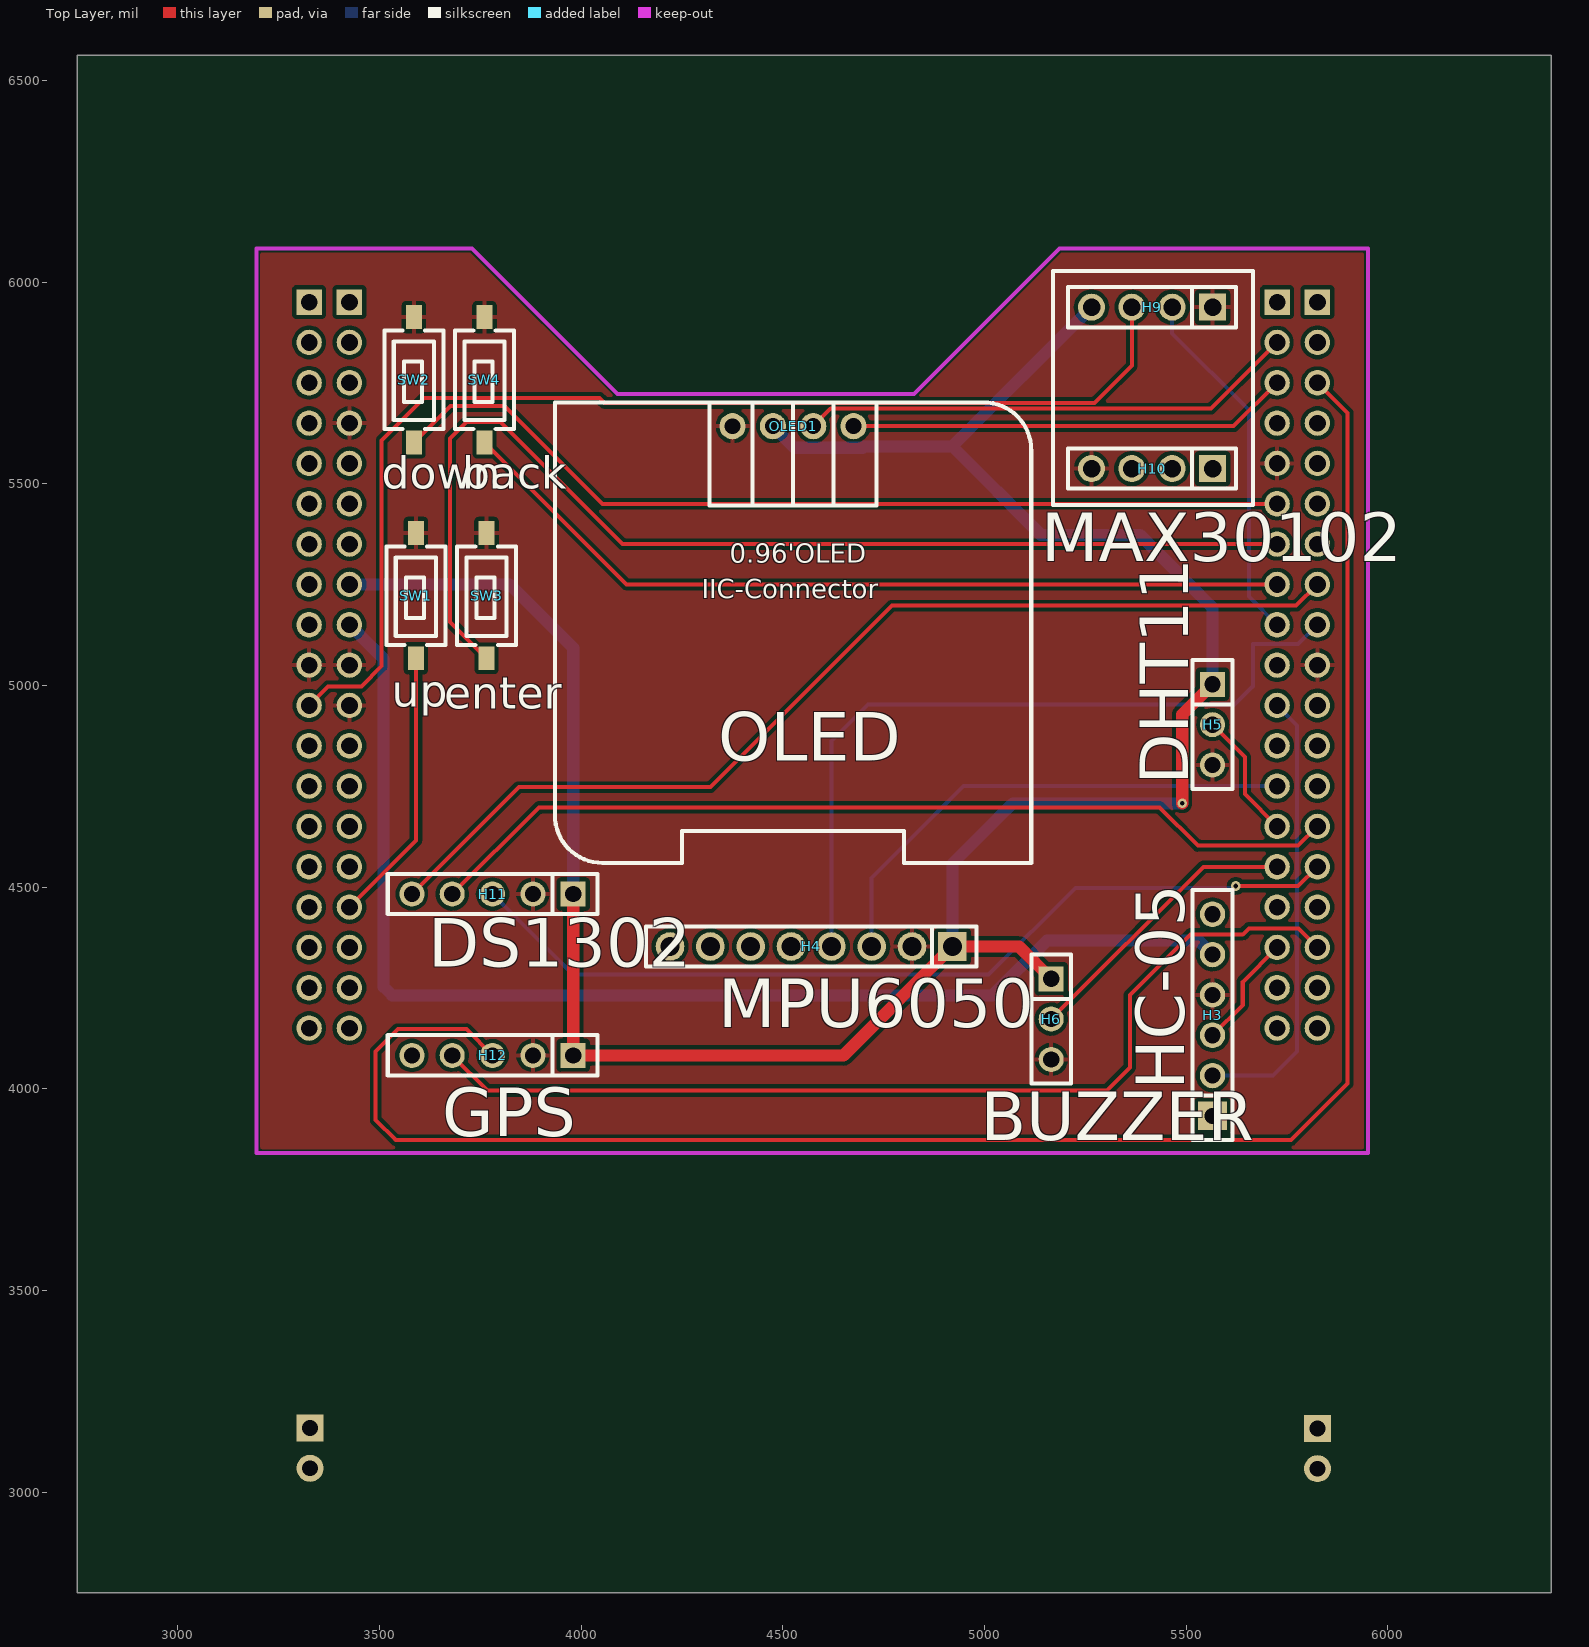
[diagram p0: Top Layer view]
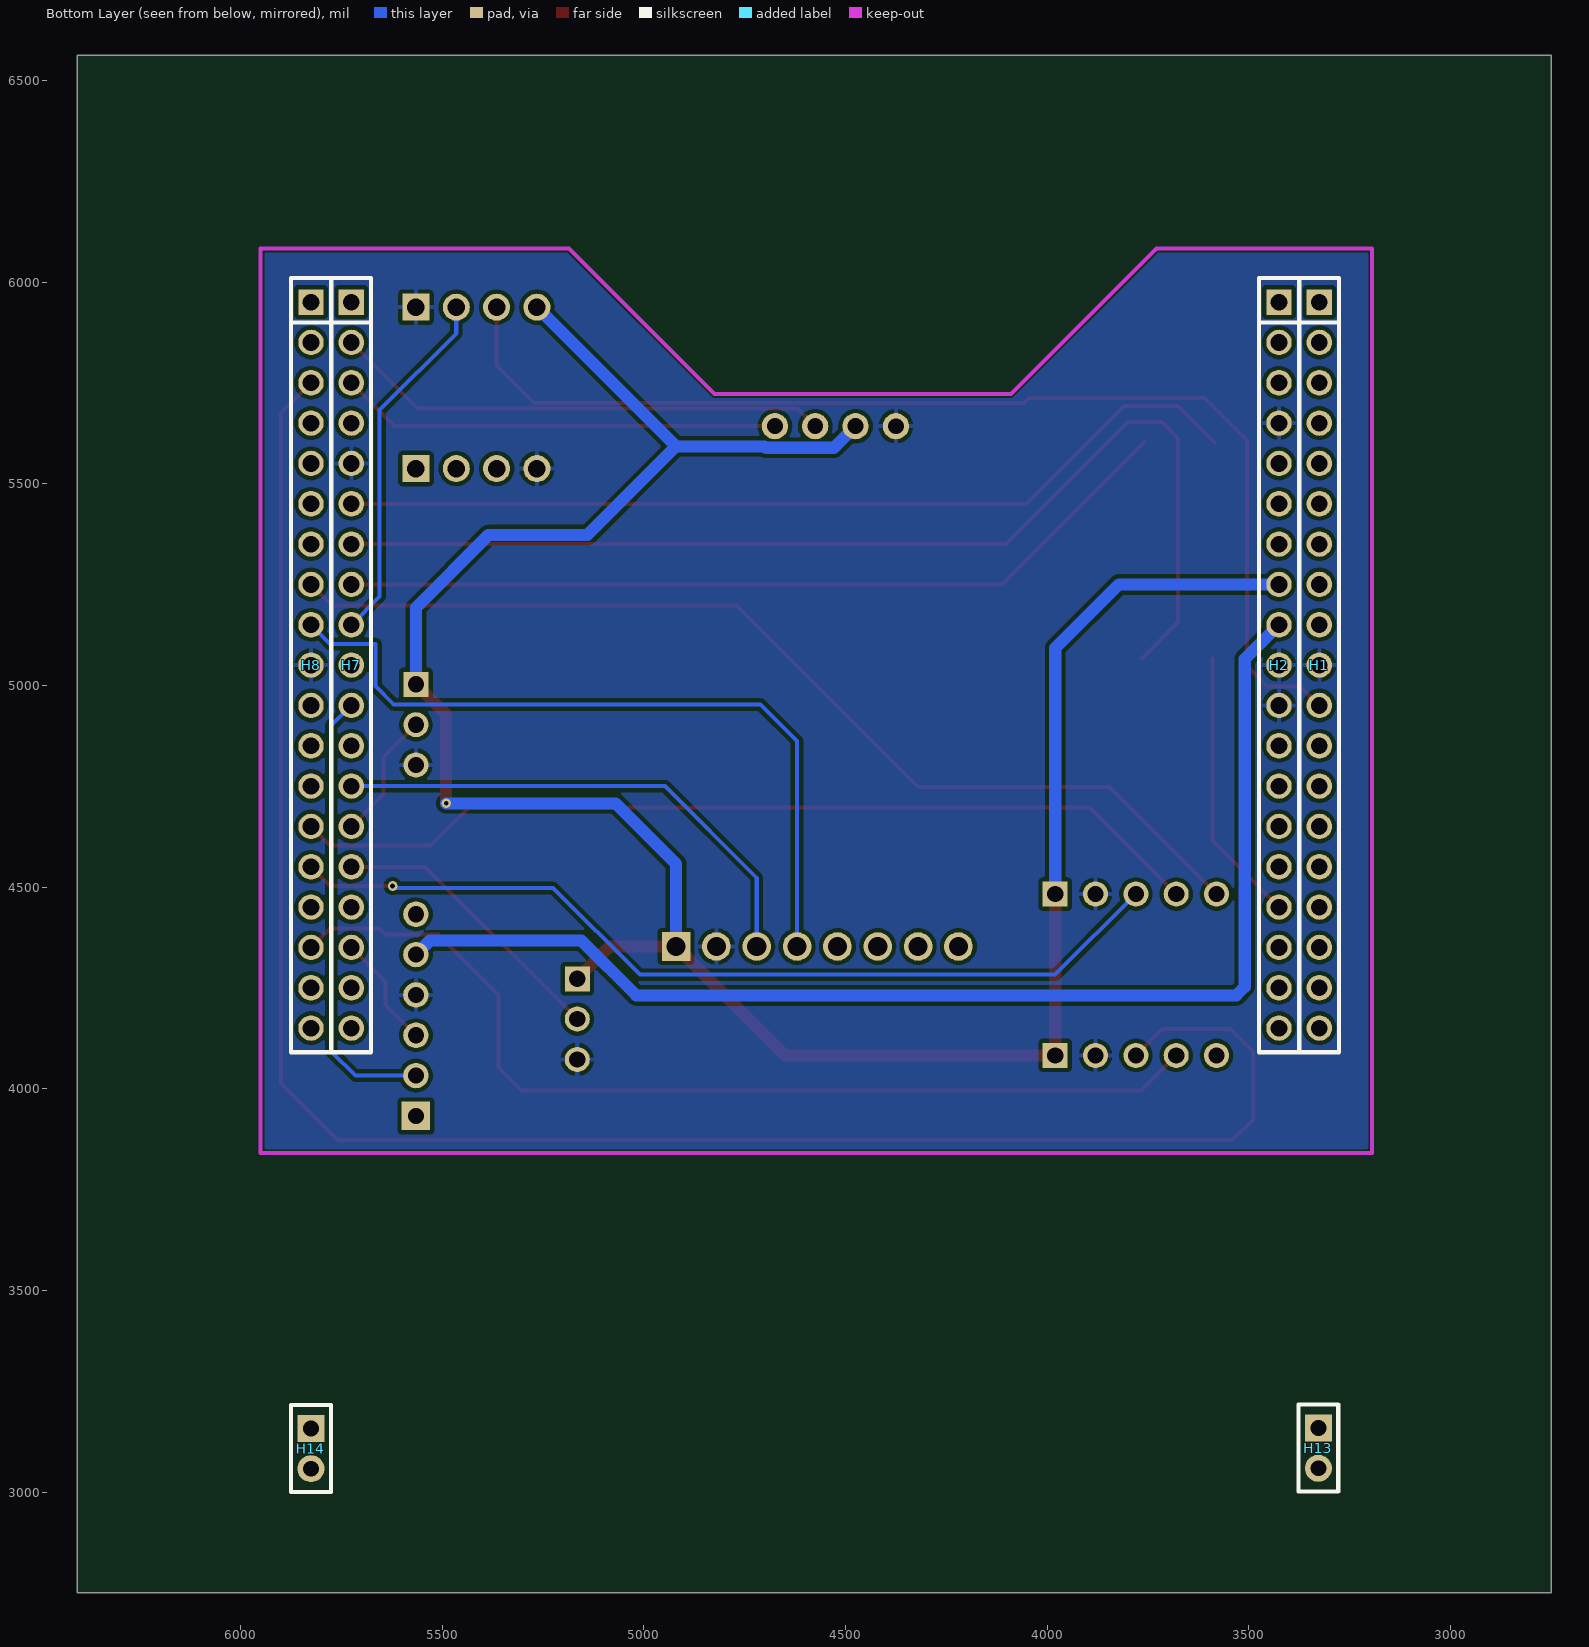
[diagram p1: Bottom Layer view, seen from below]
# Altium PCB MISC49932.pcbdoc
Units mil, origin at the board's own origin, x right, y up, seen from the top; angles counter-clockwise.
Board outline 3655 x 3812.56 mil, 2 copper layers (Top Layer, Bottom Layer), stack 62.206 mil thick; 19 components, 75 nets, 130 pads, 2 vias.

## Layer stack, top to bottom
Top Solder Mask Layer: solder mask 0.394, Dk 3.3
Top Layer: signal copper 1.379
Dielectric1: surface 59.449, FR4, Dk 4.5
Bottom Layer: signal copper 1.378
Bottom Solder Mask Layer: solder mask 0.394, Dk 3.3

## Board outline
6405,2750 2750,2750 2750,6562.56 6405,6562.56

## Design rules (kind name [scope] priority, off if disabled: settings)
BoardOutlineClearance copperThickness2oz_1 [All] p2 off: genericclearance=7.99 ignorepadtopadclearanceinfootprint=FALSE except(0: Arc-SplitContinuation Track-SplitContinuation SMDPad-SplitContinuation THPad-SplitContinuation Via-SplitContinuation Fill-SplitContinuation Region-SplitContinuation Poly-SplitContinuation Text-SplitContinuation Hole-SplitContinuation; 5.98: Arc-CutoutEdge SMDPad-CutoutEdge THPad-CutoutEdge Via-CutoutEdge Fill-CutoutEdge Region-CutoutEdge Text-CutoutEdge; 6.93: Hole-OutlineEdge Hole-CutoutEdge; 10: Poly-OutlineEdge Poly-CutoutEdge; 11.81: Arc-OutlineEdge Track-OutlineEdge SMDPad-OutlineEdge THPad-OutlineEdge Via-OutlineEdge Fill-OutlineEdge Region-OutlineEdge Text-OutlineEdge Track-CutoutEdge)
BoardOutlineClearance Plane_innerPlane_1 [All] p4 off: genericclearance=4.02 ignorepadtopadclearanceinfootprint=FALSE except(0: Arc-SplitContinuation Track-SplitContinuation SMDPad-SplitContinuation THPad-SplitContinuation Via-SplitContinuation Fill-SplitContinuation Region-SplitContinuation Poly-SplitContinuation Text-SplitContinuation Hole-SplitContinuation; 6: SMDPad-CutoutEdge THPad-CutoutEdge Via-CutoutEdge Fill-CutoutEdge Region-CutoutEdge Text-CutoutEdge; 6.93: Hole-OutlineEdge Hole-CutoutEdge; 10: Poly-OutlineEdge Poly-CutoutEdge; 11.8: Arc-OutlineEdge Track-OutlineEdge SMDPad-OutlineEdge THPad-OutlineEdge Via-OutlineEdge Fill-OutlineEdge Region-OutlineEdge Text-OutlineEdge; 11.81: Arc-CutoutEdge Track-CutoutEdge)
BoardOutlineClearance Copper_copperRegion_1 [All] p6 off: genericclearance=4.02 ignorepadtopadclearanceinfootprint=FALSE except(0: Arc-SplitContinuation Track-SplitContinuation SMDPad-SplitContinuation THPad-SplitContinuation Via-SplitContinuation Fill-SplitContinuation Region-SplitContinuation Poly-SplitContinuation Text-SplitContinuation Hole-SplitContinuation; 6: SMDPad-CutoutEdge THPad-CutoutEdge Via-CutoutEdge Fill-CutoutEdge Region-CutoutEdge Text-CutoutEdge; 6.93: Hole-OutlineEdge Hole-CutoutEdge; 10: Poly-OutlineEdge Poly-CutoutEdge; 11.8: Arc-OutlineEdge Track-OutlineEdge SMDPad-OutlineEdge THPad-OutlineEdge Via-OutlineEdge Fill-OutlineEdge Region-OutlineEdge Text-OutlineEdge; 11.81: Arc-CutoutEdge Track-CutoutEdge)
BoardOutlineClearance Copper_copperRegion_copperThickness1oz_1 [All] p8 off: genericclearance=4.02 ignorepadtopadclearanceinfootprint=FALSE except(0: Arc-SplitContinuation Track-SplitContinuation SMDPad-SplitContinuation THPad-SplitContinuation Via-SplitContinuation Fill-SplitContinuation Region-SplitContinuation Poly-SplitContinuation Text-SplitContinuation Hole-SplitContinuation; 6: SMDPad-CutoutEdge THPad-CutoutEdge Via-CutoutEdge Fill-CutoutEdge Region-CutoutEdge Text-CutoutEdge; 6.93: Hole-OutlineEdge Hole-CutoutEdge; 10: Poly-OutlineEdge Poly-CutoutEdge; 11.8: Arc-OutlineEdge Track-OutlineEdge SMDPad-OutlineEdge THPad-OutlineEdge Via-OutlineEdge Fill-OutlineEdge Region-OutlineEdge Text-OutlineEdge; 11.81: Arc-CutoutEdge Track-CutoutEdge)
BoardOutlineClearance Copper_copperRegion_Copper_copperRegion_1 [All] p10 off: genericclearance=4.02 ignorepadtopadclearanceinfootprint=FALSE except(0: Arc-SplitContinuation Track-SplitContinuation SMDPad-SplitContinuation THPad-SplitContinuation Via-SplitContinuation Fill-SplitContinuation Region-SplitContinuation Poly-SplitContinuation Text-SplitContinuation Hole-SplitContinuation; 6: SMDPad-CutoutEdge THPad-CutoutEdge Via-CutoutEdge Fill-CutoutEdge Region-CutoutEdge Text-CutoutEdge; 6.93: Hole-OutlineEdge Hole-CutoutEdge; 10: Poly-OutlineEdge Poly-CutoutEdge; 11.8: Arc-OutlineEdge Track-OutlineEdge SMDPad-OutlineEdge THPad-OutlineEdge Via-OutlineEdge Fill-OutlineEdge Region-OutlineEdge Text-OutlineEdge; 11.81: Arc-CutoutEdge Track-CutoutEdge)
BoardOutlineClearance copperThickness1oz_1 [All] p12: genericclearance=4.02 ignorepadtopadclearanceinfootprint=FALSE except(0: Arc-SplitContinuation Track-SplitContinuation SMDPad-SplitContinuation THPad-SplitContinuation Via-SplitContinuation Fill-SplitContinuation Region-SplitContinuation Poly-SplitContinuation Text-SplitContinuation Hole-SplitContinuation; 6: SMDPad-CutoutEdge THPad-CutoutEdge Via-CutoutEdge Fill-CutoutEdge Region-CutoutEdge Text-CutoutEdge; 6.93: Hole-OutlineEdge Hole-CutoutEdge; 10: Poly-OutlineEdge Poly-CutoutEdge; 11.8: Arc-OutlineEdge Track-OutlineEdge SMDPad-OutlineEdge THPad-OutlineEdge Via-OutlineEdge Fill-OutlineEdge Region-OutlineEdge Text-OutlineEdge; 11.81: Arc-CutoutEdge Track-CutoutEdge)
Clearance copperThickness2oz [All] p1 off: gap=7.99 ignorepadtopadclearanceinfootprint=FALSE except(5.98: SMDPad-Track SMDPad-SMDPad THPad-Track SMDPad-THPad THPad-THPad Track-Via SMDPad-Via THPad-Via Via-Via Fill-Track Region-Track Fill-SMDPad Region-SMDPad Fill-THPad Region-THPad Fill-Via Region-Via Fill-Fill Fill-Region Region-Region Arc-Track Arc-SMDPad Arc-THPad Arc-Via Fill-Arc Region-Arc Arc-Arc Text-Track SMDPad-Text Text-THPad Text-Via Fill-Text Region-Text Arc-Text Text-Text; 6.93: Hole-Track Hole-SMDPad Hole-THPad Hole-Via Fill-Hole Region-Hole Hole-Arc Hole-Text; 10: Poly-Track Poly-SMDPad Poly-THPad Poly-Via Poly-Fill Poly-Region Poly-Poly Poly-Arc Poly-Text Poly-Hole)
Clearance Plane_innerPlane [All] p3 off: gap=4.02 ignorepadtopadclearanceinfootprint=FALSE except(5.98: SMDPad-Track SMDPad-SMDPad THPad-Track SMDPad-THPad THPad-THPad Track-Via SMDPad-Via THPad-Via Via-Via Fill-Track Region-Track Fill-SMDPad Region-SMDPad Fill-THPad Region-THPad Fill-Via Region-Via Fill-Fill Fill-Region Region-Region; 6: Arc-Track Arc-SMDPad Arc-THPad Arc-Via Fill-Arc Region-Arc Arc-Arc Text-Track SMDPad-Text Text-THPad Text-Via Fill-Text Region-Text Arc-Text Text-Text; 6.93: Hole-Track Hole-SMDPad Hole-THPad Hole-Via Fill-Hole Region-Hole Hole-Arc Hole-Text; 10: Poly-Track Poly-SMDPad Poly-THPad Poly-Via Poly-Fill Poly-Region Poly-Poly Poly-Arc Poly-Text Poly-Hole)
Clearance Copper_copperRegion [All] p5 off: gap=4.02 ignorepadtopadclearanceinfootprint=FALSE except(5.98: SMDPad-Track SMDPad-SMDPad THPad-Track SMDPad-THPad THPad-THPad Track-Via SMDPad-Via THPad-Via Via-Via Fill-Track Region-Track Fill-SMDPad Region-SMDPad Fill-THPad Region-THPad Fill-Via Region-Via Fill-Fill Fill-Region Region-Region; 6: Arc-Track Arc-SMDPad Arc-THPad Arc-Via Fill-Arc Region-Arc Arc-Arc Text-Track SMDPad-Text Text-THPad Text-Via Fill-Text Region-Text Arc-Text Text-Text; 6.93: Hole-Track Hole-SMDPad Hole-THPad Hole-Via Fill-Hole Region-Hole Hole-Arc Hole-Text; 10: Poly-Track Poly-SMDPad Poly-THPad Poly-Via Poly-Fill Poly-Region Poly-Poly Poly-Arc Poly-Text Poly-Hole)
Clearance Copper_copperRegion_copperThickness1oz [All] p7 off: gap=4.02 ignorepadtopadclearanceinfootprint=FALSE except(5.98: SMDPad-Track SMDPad-SMDPad THPad-Track SMDPad-THPad THPad-THPad Track-Via SMDPad-Via THPad-Via Via-Via Fill-Track Region-Track Fill-SMDPad Region-SMDPad Fill-THPad Region-THPad Fill-Via Region-Via Fill-Fill Fill-Region Region-Region; 6: Arc-Track Arc-SMDPad Arc-THPad Arc-Via Fill-Arc Region-Arc Arc-Arc Text-Track SMDPad-Text Text-THPad Text-Via Fill-Text Region-Text Arc-Text Text-Text; 6.93: Hole-Track Hole-SMDPad Hole-THPad Hole-Via Fill-Hole Region-Hole Hole-Arc Hole-Text; 10: Poly-Track Poly-SMDPad Poly-THPad Poly-Via Poly-Fill Poly-Region Poly-Poly Poly-Arc Poly-Text Poly-Hole)
Clearance Copper_copperRegion_Copper_copperRegion [All] p9 off: gap=4.02 ignorepadtopadclearanceinfootprint=FALSE except(5.98: SMDPad-Track SMDPad-SMDPad THPad-Track SMDPad-THPad THPad-THPad Track-Via SMDPad-Via THPad-Via Via-Via Fill-Track Region-Track Fill-SMDPad Region-SMDPad Fill-THPad Region-THPad Fill-Via Region-Via Fill-Fill Fill-Region Region-Region; 6: Arc-Track Arc-SMDPad Arc-THPad Arc-Via Fill-Arc Region-Arc Arc-Arc Text-Track SMDPad-Text Text-THPad Text-Via Fill-Text Region-Text Arc-Text Text-Text; 6.93: Hole-Track Hole-SMDPad Hole-THPad Hole-Via Fill-Hole Region-Hole Hole-Arc Hole-Text; 10: Poly-Track Poly-SMDPad Poly-THPad Poly-Via Poly-Fill Poly-Region Poly-Poly Poly-Arc Poly-Text Poly-Hole)
Clearance copperThickness1oz [All] p11: gap=4.02 ignorepadtopadclearanceinfootprint=FALSE except(5.98: SMDPad-Track SMDPad-SMDPad THPad-Track SMDPad-THPad THPad-THPad Track-Via SMDPad-Via THPad-Via Via-Via Fill-Track Region-Track Fill-SMDPad Region-SMDPad Fill-THPad Region-THPad Fill-Via Region-Via Fill-Fill Fill-Region Region-Region; 6: Arc-Track Arc-SMDPad Arc-THPad Arc-Via Fill-Arc Region-Arc Arc-Arc Text-Track SMDPad-Text Text-THPad Text-Via Fill-Text Region-Text Arc-Text Text-Text; 6.93: Hole-Track Hole-SMDPad Hole-THPad Hole-Via Fill-Hole Region-Hole Hole-Arc Hole-Text; 10: Poly-Track Poly-SMDPad Poly-THPad Poly-Via Poly-Fill Poly-Region Poly-Poly Poly-Arc Poly-Text Poly-Hole)
DiffPairsRouting differentialPair [All] p1: maxlimit=6 minlimit=6 mostfreqgap=6 toplayer_minwidth=5 toplayer_prefwidth=10 toplayer_maxwidth=100 toplayer_mingap=6 toplayer_prefgap=6 toplayer_maxgap=6 bottomlayer_minwidth=5 bottomlayer_prefwidth=10 bottomlayer_maxwidth=100 bottomlayer_mingap=6 bottomlayer_prefgap=6 bottomlayer_maxgap=6 maxuncoupledlength=10
HoleToHoleClearance otherClearance [All] p1: gap=11.81 allowstackedmicrovias=TRUE
Length netLength [All] p1: minlimit=0 maxlimit=0
PasteMaskExpansion pasteMaskExpansion [All] p1: expansion=0
PlaneConnect innerPlane [All] p1: planeconnectstyle=Relief reliefexpansion=20 reliefentries=4 reliefconductorwidth=10 reliefairgap=10
PolygonConnect copperRegion_copperThickness1oz [All] p1 off: connectstyle=Relief reliefconductorwidth=10 reliefentries=4 polygonreliefangle="90 Angle" airgapwidth=10 via.connectstyle=Relief via.reliefconductorwidth=10 via.reliefentries=4 via.polygonreliefangle="90 Angle" via.airgapwidth=10
PolygonConnect copperRegion_Copper_copperRegion [All] p2 off: connectstyle=Relief reliefconductorwidth=10 reliefentries=4 polygonreliefangle="90 Angle" airgapwidth=10 via.connectstyle=Relief via.reliefconductorwidth=10 via.reliefentries=4 via.polygonreliefangle="90 Angle" via.airgapwidth=10
PolygonConnect copperRegion [All] p3: connectstyle=Relief reliefconductorwidth=10 reliefentries=4 polygonreliefangle="90 Angle" airgapwidth=10 via.connectstyle=Relief via.reliefconductorwidth=10 via.reliefentries=4 via.polygonreliefangle="90 Angle" via.airgapwidth=10
RoutingVias viaSize [All] p1: holewidth=12.01 width=24.02 viastyle="Through Hole" minholewidth=11.81 minwidth=19.68 maxholewidth=248.03 maxwidth=393.7
SolderMaskExpansion solderMaskExpansion [IsVia] p1: expansion=-1000 istentingtop=TRUE
SolderMaskExpansion solderMaskExpansion [All] p2: expansion=2 istentingtop=FALSE
Width copperThickness2oz_2 [All] p1 off: maxlimit=100 minlimit=8 preferedwidth=10
Width copperThickness1oz_2 [All] p2: maxlimit=100 minlimit=5 preferedwidth=10

## Components (designator, comment, footprint, x,y, rotation, side; value= is the part's Value field where it differs from the comment)
H1 "C2897382" HDR-TH_19P-P2.54-V-F 3325.16,5050.22 r270 bottom locked
H2 "C2897382" HDR-TH_19P-P2.54-V-F 3425.16,5050.22 r270 bottom locked
H3 "" HDR-TH_6P-P2.54-V-F 5565,4182.56 r90 top
H4 "" HDR-TH_8P-P2.54-V-F-1 4570,4352.56 r180 top
H5 "" HDR-TH_3P-P2.54-V-F 5565,4902.56 r270 top
H6 "" HDR-TH_3P-P2.54-V-F 5165,4172.56 r270 top
H7 "C2897382" HDR-TH_19P-P2.54-V-F 5725.16,5050.22 r270 bottom locked
H8 "C2897382" HDR-TH_19P-P2.54-V-F 5825.16,5050.22 r270 bottom locked
H9 "" HDR-TH_4P-P2.54-V-F 5415,5937.56 r180 top
H10 "" HDR-TH_4P-P2.54-V-F 5415,5537.56 r180 top
H11 "" HDR-TH_5P-P2.54-V-F 3780,4482.56 r180 top
H12 "" HDR-TH_5P-P2.54-V-F 3780,4082.56 r180 top
H13 "" HDR-TH_2P-P2.54-V-F 3327.44,3108.94 r270 bottom locked
H14 "" HDR-TH_2P-P2.54-V-F 5825.32,3107.87 r270 bottom locked
OLED1 "" 0.96OLED_4P 4525,5642.56 r0 top
SW1 "" Key_SMD_3.6x6.1x2.5 3590,5222.56 r90 top
SW2 "" Key_SMD_3.6x6.1x2.5 3585,5757.56 r90 top
SW3 "" Key_SMD_3.6x6.1x2.5 3765,5222.56 r90 top
SW4 "" Key_SMD_3.6x6.1x2.5 3760,5757.56 r90 top

## Footprints (in the part's own frame and the unit in brackets; to place one, negate y for a bottom-side part, rotate by r counter-clockwise, add the part's x,y. Pads: shape width x height; smd on the part's side, far side on the other; paste and mask are expansions set on the pad)
0.96OLED_4P [mm]
  round 1.65 hole 1 copper offset 0,0: 1(-3.81,-0.001) 2(-1.27,0.002) 3(1.27,0.002) 4(3.81,0.002)
  silkscreen extent -15,-27.5 15,1.5
HDR-TH_2P-P2.54-V-F [mm]
  rect 1.7x1.7 hole 1: 1(-1.27,0)
  round 1.7 hole 1: 2(1.27,0)
  silkscreen extent -2.74,-1.25 2.74,1.25
HDR-TH_3P-P2.54-V-F [mil]
  rect 62x62 hole 40.16: 1(-100,0)
  round 62 hole 40.16: 2(0,0) 3(100,0)
  silkscreen extent -160,-49 160,49
HDR-TH_4P-P2.54-V-F [mm]
  rect 1.7x1.7 hole 1.1: 1(-3.81,0)
  round 1.7 hole 1.1: 2(-1.27,0) 3(1.27,0) 4(3.81,0)
  silkscreen extent -5.29,-1.27 5.29,1.27
HDR-TH_5P-P2.54-V-F [mil]
  rect 62x62 hole 40.16: 1(-200,0)
  round 62 hole 40.16: 2(-100,0) 3(0,0) 4(100,0) 5(200,0)
  silkscreen extent -260,-50 260,50
HDR-TH_6P-P2.54-V-F [mm]
  rect 1.8x1.8 hole 1.02: 1(-6.35,0)
  round 1.6 hole 1.02: 2(-3.81,0) 3(-1.27,0) 4(1.27,0) 5(3.81,0) 6(6.35,0)
  silkscreen extent -7.87,-1.25 7.87,1.25
HDR-TH_8P-P2.54-V-F-1 [mm]
  rect 1.8x1.8 hole 1.2: 1(-8.89,0)
  round 1.8 hole 1.2: 2(-6.35,0) 3(-3.81,0) 4(-1.27,0) 5(1.27,0) 6(3.81,0) 7(6.35,0) 8(8.89,0)
  silkscreen extent -10.41,-1.25 10.41,1.25
HDR-TH_19P-P2.54-V-F [mm]
  rect 1.6x1.6 hole 1.05: 1(-22.86,0)
  round 1.6 hole 1.05: 2(-20.32,0) 3(-17.78,0) 4(-15.24,0) 5(-12.7,0) 6(-10.16,0) 7(-7.62,0) 8(-5.08,0) 9(-2.54,0) 10(0,0) 11(2.54,0) 12(5.08,0) 13(7.62,0) 14(10.16,0) 15(12.7,0) 16(15.24,0) 17(17.78,0) 18(20.32,0) 19(22.86,0)
  silkscreen extent -24.38,-1.25 24.38,1.25
Key_SMD_3.6x6.1x2.5 [mil]
  rect 59.1x39.4 smd paste+0 mask+2: 1(-155.5,0) 2(155.5,0)
  silkscreen extent -122,-73 122,73

## Via types
v1: diameter 24.02, hole 12, Top Layer to Bottom Layer, 2 vias

## Nets (pads, with @x,y where several pads share a name; then routed paths per layer and width w, separated by ;. In a path a pad name is that pad's centre, name@x,y a point inside that pad or via, vN(x,y) a via of type N, cw(c..) or ccw(c..) an arc to the next point about the centre after c; other vN are vias at no path point)
+3V3: H2.8 H4.1 H5.1 H6.1 H9.4 H11.1 H12.1 OLED1.2 | length 6080.5
  Top Layer w30: H11.1 H12.1 4650,4082.56 H4.1 5085,4352.56 H6.1 ; v1(5490,4707.56) 5490,4927.56 H5.1
  Bottom Layer w30: H2.8 3822.35,5250.22 3980,5092.56 H11.1 ; OLED1.2 4528.46,5589.15 4697.15,5589.15 4700.56,5592.56 4920,5592.56 ; H4.1 4920,4557.56 5070,4707.56 v1(5490,4707.56) ; H9.4 4920,5592.56 ; H5.1 5565,5192.56 5385,5372.56 5140,5372.56 4920,5592.56
+5V: H2.9 H3.5 | length 3067.5
  Bottom Layer w30: H2.9 3510,5065.38 3510,4252.56 3531.21,4231.35 5018.79,4231.35 5155,4367.56 5530,4367.56 H3.5
ADO: H4.7
AGND: H8.16
AVDD: H7.4
BOOT0: H1.4
CLK: H8.15 H11.3 | length 2238.8
  Top Layer w10: v1@5622.78,4502.56 5777.5,4502.56 H8.15
  Bottom Layer w10: H11.3 3980,4282.56 5010,4282.56 5225,4497.56 5617.78,4497.56 v1(5622.74,4502.52)
DAT: H8.14 H11.4 | length 2293.3
  Top Layer w10: H11.4 3895,4697.56 5433.54,4697.56 5528.54,4602.56 5777.5,4602.56 H8.14
E5V: H2.3
EN: H3.6
GND: H1.10 H2.4 H2.10 H2.11 H3.4 H4.2 H5.3 H6.3 H7.5 H8.10 H9.1 H10.4 H11.2 H12.2 OLED1.1 SW1.2 SW2.2 SW3.2 SW4.2
INT: H4.8
IOREF: H2.6
NC: H8.5
PA0: H2.14
PA1: H2.15
PA2: H7.18
PA3: H7.19
PA4: H2.16 SW1.1 | length 685.1
  Top Layer w10: H2.16 3590,4615.06 SW1.1
PA5: H7.6 SW2.1 | length 2278
  Top Layer w10: SW2.1 3675.5,5692.56 3810,5692.56 4052.35,5450.22 H7.6
PA6: H7.7 SW3.1 | length 2774.7
  Top Layer w10: SW3.1 3675,5157.06 3675,5612.56 3715,5652.56 3800,5652.56 4102.35,5350.22 H7.7
PA7: H7.8 SW4.1 | length 2110.9
  Top Layer w10: SW4.1 4111.85,5250.22 H7.8
PA8: H7.12
PA9: H3.2 H7.11 | length 1113.2
  Bottom Layer w10: H3.2 5715,4032.56 5775,4092.56 5775,4900.38 H7.11
PA10: H3.3 H7.17 | length 284
  Top Layer w10: H3.3 5640,4207.56 5640,4265.06 H7.17
PA11: H8.7
PA12: H8.6
PA13: H1.7
PA14: H1.8
PA15: H1.9
PB0: H2.17
PB1: H8.12
PB2: H8.11
PB3: H7.16
PB4: H5.2 H7.14 | length 318.7
  Top Layer w10: H5.2 5645,4822.56 5645,4730.38 H7.14
PB5: H6.2 H7.15 | length 716.6
  Top Layer w10: H6.2 5542.65,4550.22 H7.15
PB6: H7.9 H9.2 | length 895.1
  Bottom Layer w10: H9.2 5465,5872.56 5655,5682.56 5655,5220.38 H7.9
PB7: H1.11 H9.3 | length 2872.1
  Top Layer w10: H1.11 3372.5,4997.56 3455,4997.56 3505,5047.56 3505,5607.56 3610,5712.56 4045,5712.56 4057.47,5700.09 5272.53,5700.09 5365,5792.56 H9.3
PB8: H7.2 OLED1.3 | length 1236.2
  Top Layer w10: OLED1.3 4618.46,5686.08 5561.02,5686.08 H7.2
PB9: H7.3 OLED1.4 | length 1094.7
  Top Layer w10: OLED1.4 5617.55,5642.61 H7.3
PB10: H4.3 H7.13 | length 1269.5
  Bottom Layer w10: H4.3 4720,4522.56 4947.65,4750.22 H7.13
PB11: H4.4 H8.9 | length 1895.2
  Bottom Layer w10: H4.4 4620,4861.76 4710.8,4952.56 5620,4952.56 5665.28,4997.84 5665.28,5102.56 5777.5,5102.56 H8.9
PB12: H8.8 H11.5 | length 2563.1
  Top Layer w10: H11.5 3845,4747.56 4320,4747.56 4770,5197.56 5772.5,5197.56 H8.8
PB15: H8.13
PC0: H2.19
PC1: H2.18
PC2: H1.18
PC3: H1.19
PC4: H8.17 H12.4 | length 2472.8
  Top Layer w10: H12.4 3767.07,3995.49 5302.93,3995.49 5360,4052.56 5360,4232.56 5510,4382.56 5640,4382.56 5655,4397.56 5777.81,4397.56 H8.17
PC5: H8.3 H12.3 | length 4767.1
  Top Layer w10: H12.3 3715,4147.56 3545,4147.56 3490,4092.56 3490,3922.56 3540,3872.56 5760,3872.56 5900,4012.56 5900,5675.38 H8.3
PC6: H8.2
PC7: H7.10
PC8: H8.1
PC9: H7.1
PC10: H1.1
PC11: H2.1
PC12: H1.2
PC13: H1.12
PC14: H1.13
PC15: H1.14
PD2: H2.2
PF0: H1.15
PF1: H1.16
PF4: H8.19
PF5: H8.18
PF6: H1.5
PF7: H1.6
RESET: H2.7
STATE: H3.1
U5V: H8.4
VBAT: H1.17
VDD: H1.3
VIN: H2.12
XCL: H4.6
XDA: H4.5
pads on no net: H2.5 H2.13 H10.1 H10.2 H10.3 H12.5 H13.1 H13.2 H14.1 H14.2

## Polygon pours and split planes (outlines as drawn)
GND on Bottom Layer (solid, remove dead copper, pour order 2): 3035,6312.56 3035,3712.56 6110,3712.56 6110,6312.56
GND on Top Layer (solid, remove dead copper, pour order 0): 3000,6282.56 3000,3727.56 6155,3727.56 6155,6282.56

## Keep-outs
Board Outline Layer:
  lines w10: 3194.25,3840.22 5950.16,3840.22 5950.16,6083.25 5185.69,6083.25 4825,5722.56 4090,5722.56 3729.31,6083.25 3194.25,6083.25 3194.25,3840.22

## Silkscreen, mask and mechanical layers (free items; w line width, h text height)
Top Silkscreen Layer:
  lines w10: 5170,5447.56 5665,5447.56 5665,6027.56 5170,6027.56 5170,5447.56
  text "down" at 3505,5487.56 h80
  text "back" at 3705,5487.56 h80
  text "MAX30102" at 5140,5307.56 h120
  text "up" at 3530,4947.56 h80
  text "enter" at 3660,4942.56 h80
  text "OLED" at 4340,4812.56 h120
  text "DHT11" at 5505,4753.37 h120 r90
  text "DS1302" at 3620,4302.56 h120
  text "MPU6050" at 4340,4152.56 h120
  text "HC-05" at 5495,3997.56 h120 r90
  text "GPS" at 3655,3882.56 h120
  text "BUZZER" at 4990,3872.56 h120